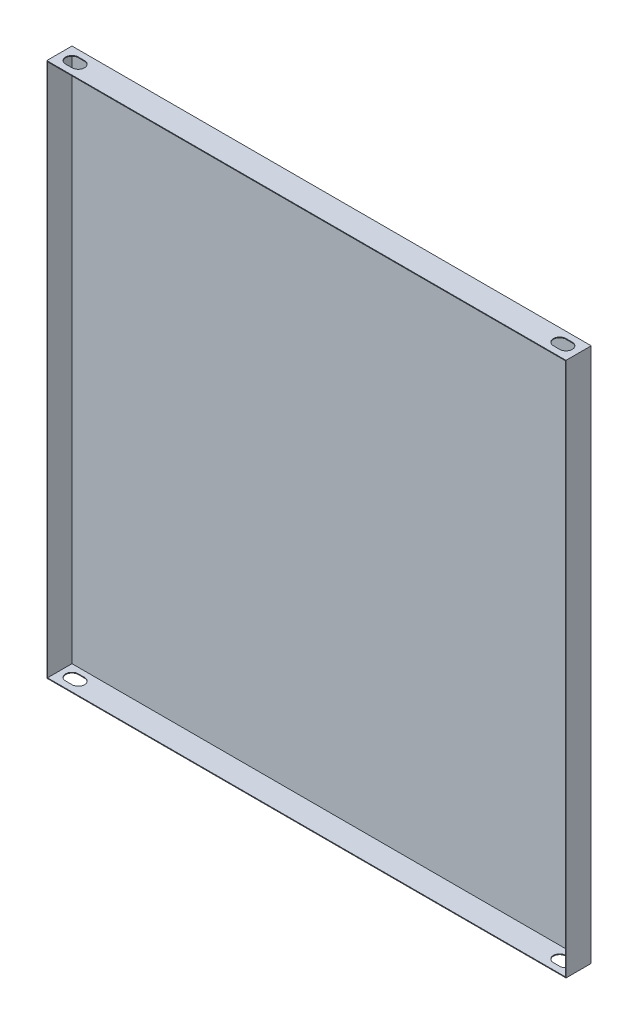
SolidWorks part; units mm, degrees
material "SPHC"
ref_plane "Front Plane" through (0, 0, 0) normal (0, 0, 1) x (1, 0, 0)
ref_plane "Top Plane" through (0, 0, 0) normal (0, 1, 0) x (1, 0, 0)
ref_plane "Right Plane" through (0, 0, 0) normal (1, 0, 0) x (0, 0, -1)
sketch "Sketch1" plane through (0, 0, 0) normal (0, 0, 1) x (1, 0, 0)
  line L1 (-825, 850) -> (825, 850)
  line L2 (-825, 850) -> (-825, -850)
  line L3 (-825, -850) -> (825, -850)
  line L4 (825, 850) -> (825, -850)
  line L5 (-825, 850) -> (825, -850) construction
  line L6 (-825, -850) -> (825, 850) construction
  point P0 (0, 0)
  dimension "D1" = 1650
  dimension "D2" = 1700
extrude "Boss-Extrude1" add sketch "Sketch1" along normal blind 80
shell "Shell1" thickness 2.3
sketch "Sketch2" plane through (0, -850, 0) normal (0, -1, 0) x (1, 0, 0)
  line L0 (-785, 40) -> (-765, 40) construction
  line L1 (-785, 60) -> (-765, 60)
  line L2 (-785, 20) -> (-765, 20)
  line L3 (-825, 80) -> (-825, 0) construction
  line L4 (-825, 80) -> (825, 80) construction
  line L5 (0, 0) -> (0, 80) construction
  line L6 (785, 40) -> (765, 40) construction
  line L7 (785, 60) -> (765, 60)
  line L8 (785, 20) -> (765, 20)
  arc A0 (-785, 60) -> (-785, 20) centre (-785, 40) ccw
  arc A1 (-765, 20) -> (-765, 60) centre (-765, 40) ccw
  arc A2 (785, 60) -> (785, 20) centre (785, 40) cw
  arc A3 (765, 20) -> (765, 60) centre (765, 40) cw
  point P2 (-775, 40)
  point P16 (775, 40)
  dimension "D1" = 20
  dimension "D4" = 40
  dimension "D2" = 20
  dimension "D3" = 50
extrude "Cut-Extrude1" cut sketch "Sketch2" against normal through all
